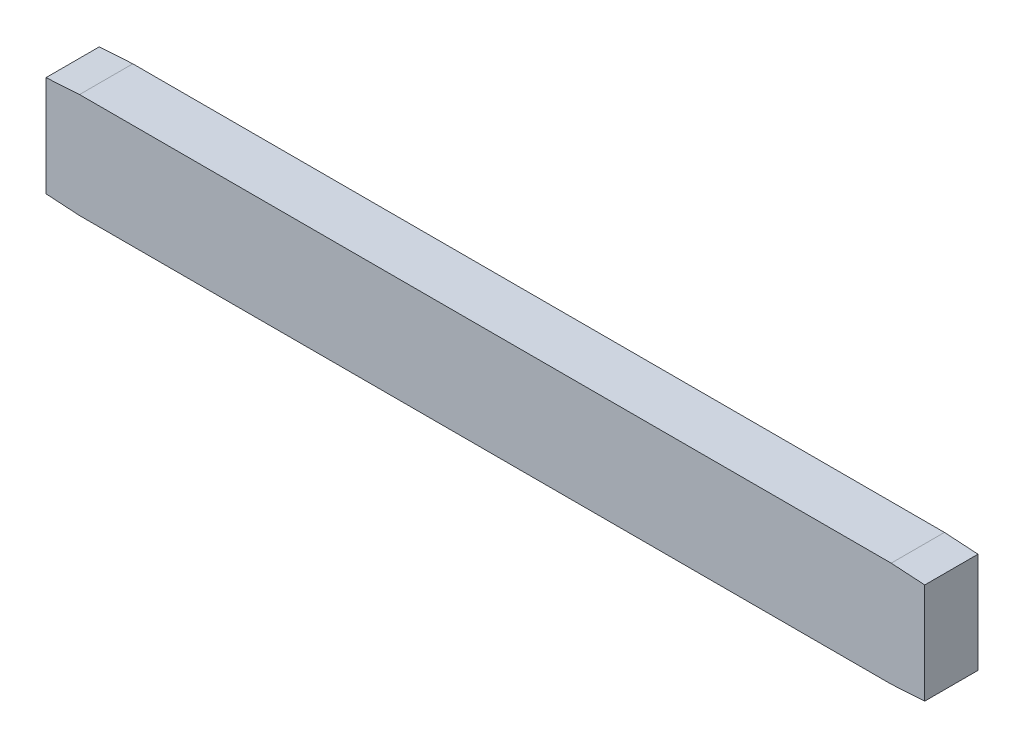
SolidWorks part; units mm, degrees
material "Q235B"
ref_plane "Front Plane" through (0, 0, 0) normal (0, 0, 1) x (1, 0, 0)
ref_plane "Top Plane" through (0, 0, 0) normal (0, 1, 0) x (1, 0, 0)
ref_plane "Right Plane" through (0, 0, 0) normal (1, 0, 0) x (0, 0, -1)
sketch "Sketch1" plane through (0, 0, 0) normal (0, 0, 1) x (1, 0, 0)
  line L0 (0, 83.5625) -> (0, -44.2168) construction
  line L1 (-104.775, 12.5) -> (104.775, 12.5)
  line L2 (-104.775, 12.5) -> (-104.775, -12.5)
  line L3 (-104.775, -12.5) -> (104.775, -12.5)
  line L4 (104.775, 12.5) -> (104.775, -12.5)
  line L5 (-140.8764, 0) -> (136.2519, 0) construction
  dimension "D1" = 25
  dimension "D2" = 209.55
extrude "Extrude1" add sketch "Sketch1" along normal mid plane 12.7
sketch "Sketch2" plane through (0, 0, 6.35) normal (0, 0, 1) x (1, 0, 0)
  line L0 (-104.775, 12) -> (-96.775, 12.5)
  line L1 (-104.775, 12.5) -> (-104.775, -12.5) construction
  line L2 (104.775, 12.5) -> (-104.775, 12.5) construction
  line L3 (-96.775, 12.5) -> (-104.775, 12.5)
  line L4 (-104.775, 12.5) -> (-104.775, 12)
  line L5 (0, 0) -> (0, 24.6393) construction
  line L6 (0, 0) -> (34.2031, 0) construction
  line L7 (96.775, 12.5) -> (104.775, 12.5)
  line L8 (104.775, 12.5) -> (104.775, 12)
  line L9 (104.775, 12) -> (96.775, 12.5)
  line L10 (104.775, -12.5) -> (104.775, -12)
  line L11 (96.775, -12.5) -> (104.775, -12.5)
  line L12 (104.775, -12) -> (96.775, -12.5)
  line L13 (-96.775, -12.5) -> (-104.775, -12.5)
  line L14 (-104.775, -12.5) -> (-104.775, -12)
  line L15 (-104.775, -12) -> (-96.775, -12.5)
  dimension "D1" = 8
  dimension "D2" = 0.5
extrude "Cut-Extrude1" cut sketch "Sketch2" against normal through all
